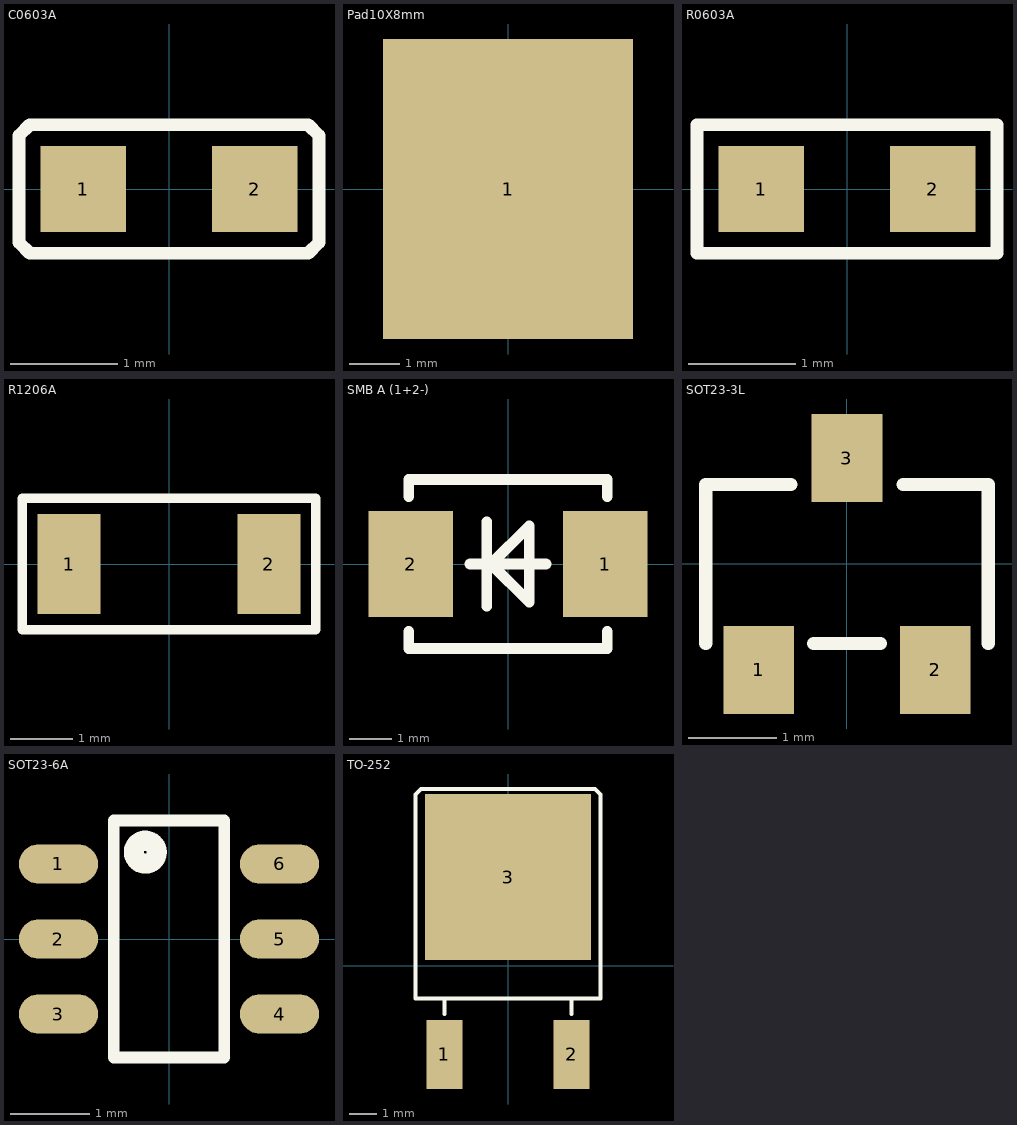
[diagram p0: the footprints below, top view; thin cyan lines are the x and y axes]
# Altium footprint library MISC82045.PcbLib: 8 footprints
Each footprint in its own frame and in the unit in brackets; x right, y up, seen from the top. Pads: shape width x height; smd on the part's side, far side on the other; paste and mask are expansions set on the pad; w line width, h text height; cw(c..) or ccw(c..) is an arc to the next point about the centre after c.

## C0603A [mm] "SMD capacitor"
pads (2):
  rect 0.8x0.8 smd mask+0.08: 1(-0.8,0) 2(0.8,0)
Top Overlay:
  lines w0.12: 0.551,-0.6 1.2,-0.6 ; -1.4,-0.5 -1.4,0.5 -1.3,0.6 1.3,0.6 1.4,0.5 1.4,-0.5 1.3,-0.6 -1.3,-0.6 -1.4,-0.5

## Pad10X8mm [mm]
pads (1):
  rect 5x6 smd: 1(0,0)

## R0603A [mm] "SMD resistor"
height 0.5
pads (2):
  rect 0.8x0.8 smd mask+0.08: 1(-0.8,0) 2(0.8,0)
Top Overlay:
  lines w0.12: -1.4,-0.6 1.4,-0.6 1.4,0.6 -1.4,0.6 -1.4,-0.6

## R1206A [mm] "SMD resistor"
pads (2):
  rect 1x1.6 smd: 1(-1.6,0) 2(1.6,0)
Top Overlay:
  lines w0.15: -2.35,-1.05 -2.35,1.05 2.35,1.05 2.35,-1.05 -2.35,-1.05

## SMB A (1+2-) [mm] "SMD diode"
pads (2):
  rect 2x2.5 smd: 1(2.3,0) 2(-2.3,0)
Top Overlay:
  lines w0.254: -2.35,-1.6 -2.35,-2 2.35,-2 2.35,-1.6 ; -2.35,1.6 -2.35,2 2.35,2 2.35,1.6 ; -0.9,0 0.9,0 ; -0.5,-1 -0.5,1 ; -0.4,0 0.5,-0.9 0.5,0.9 -0.4,0

## SOT23-3L [mm] "SMD IMOS"
pads (3):
  rect 0.8x1 smd: 1(-1,-1.2) 2(1,-1.2) 3(0,1.2)
Top Overlay:
  lines w0.15: -1.6,-0.9 -1.6,0.9 -0.635,0.9 ; -0.381,-0.9 0.381,-0.9 ; 0.635,0.9 1.6,0.9 1.6,-0.9

## SOT23-6A [mm]
pads (6):
  oval 1x0.5 smd mask+0.05: 1(-1.4,0.95) 2(-1.4,0) 3(-1.4,-0.95) 4(1.4,-0.95) 5(1.4,0) 6(1.4,0.95)
Top Overlay:
  circle w0.254: c-0.3,1.1 r0.146
  lines w0.15: -0.7,-1.5 -0.7,1.5 0.7,1.5 0.7,-1.5 -0.7,-1.5

## TO-252 [mm]
height 1.75
pads (3):
  rect 1.3x2.5 smd: 1(-2.3,-3.212) 2(2.3,-3.212)
  rect 6x6 smd: 3(0,3.213)
Top Overlay:
  lines w0.15: -2.3,-1.75 -2.3,-1.18 ; 2.3,-1.75 2.3,-1.18 ; -3.35,-1.18 3.35,-1.18 3.35,6.19 3.35,6.2 3.15,6.4 -3.15,6.4 -3.35,6.2 -3.35,-1.18